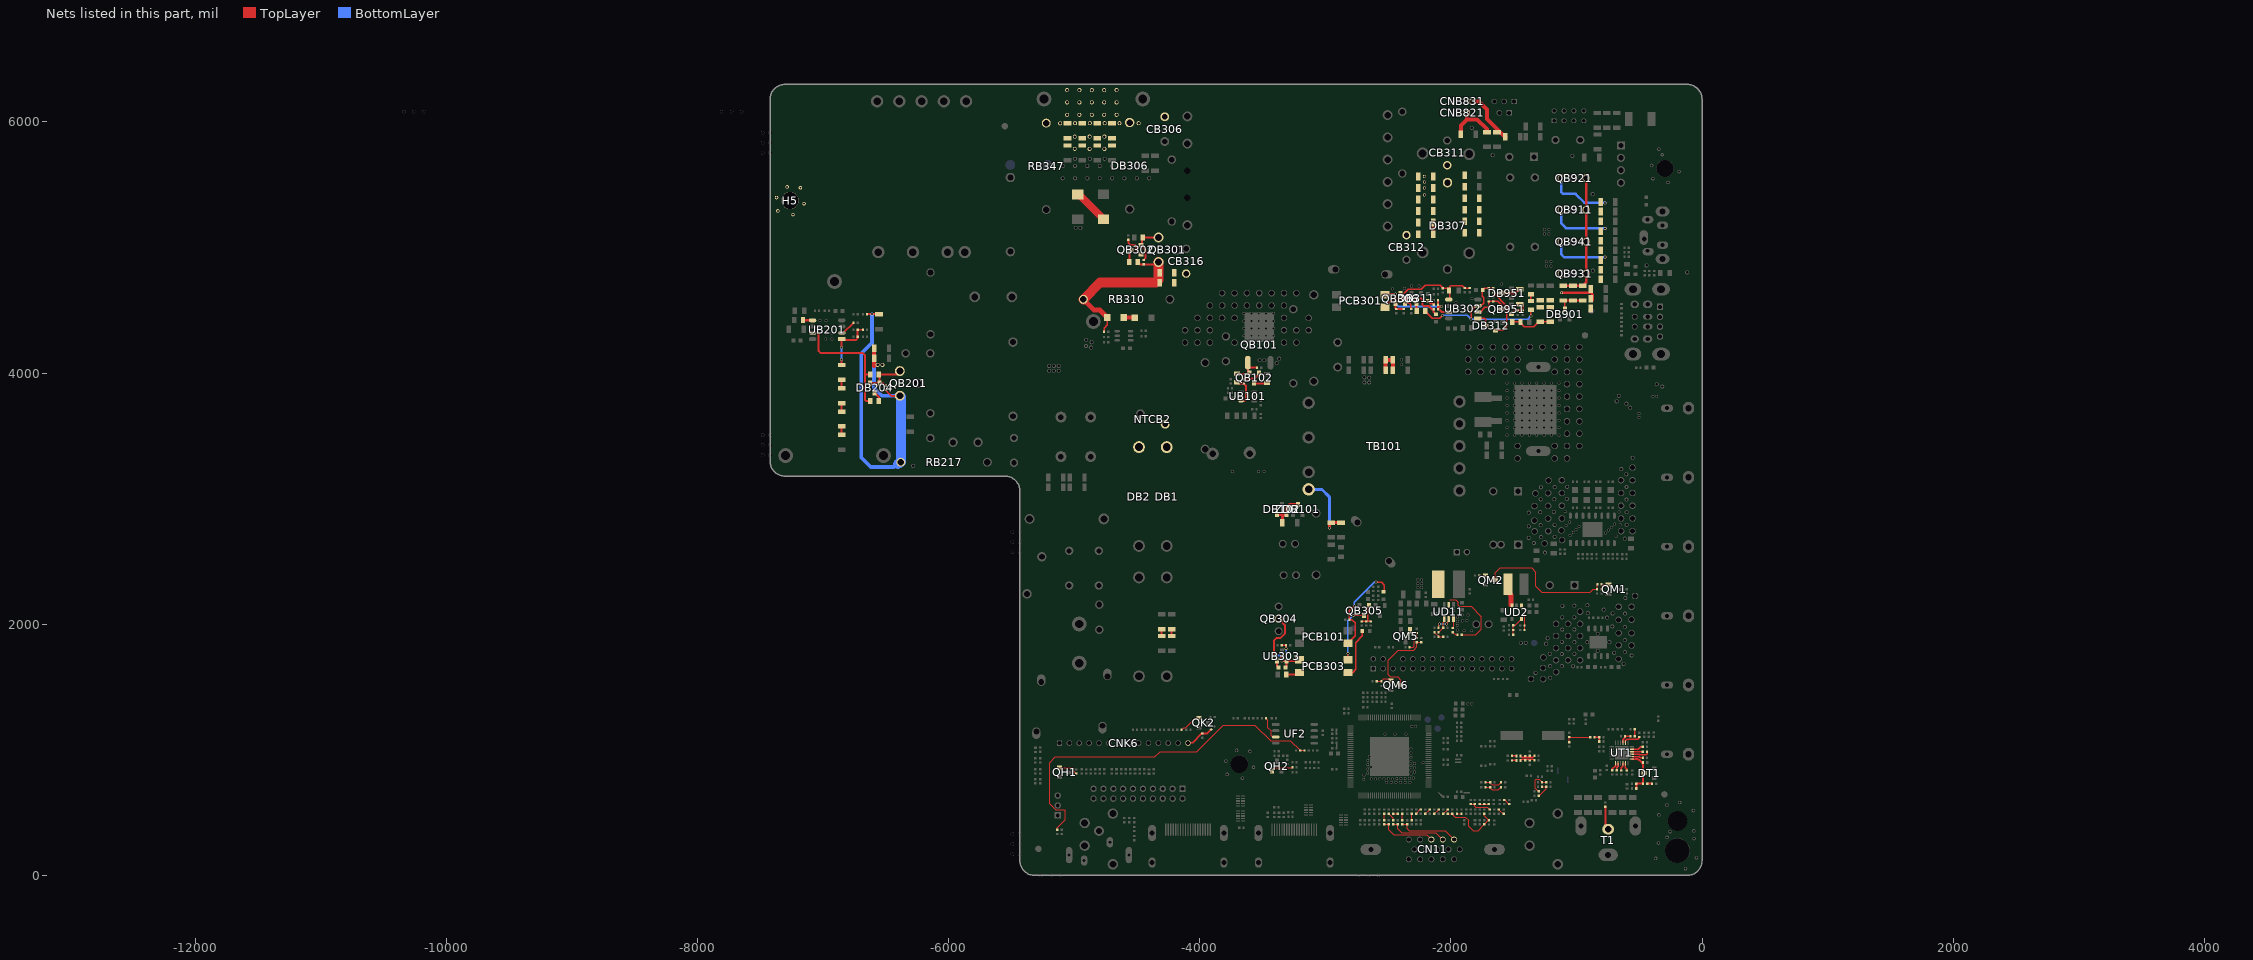
[diagram p0: the nets of this part, all layers, seen from the top]
# Altium PCB MISC84277.PcbDoc (part 12 of 15)
Units mil, origin at the board's own origin, x right, y up, seen from the top; angles counter-clockwise.
Board outline 7422.08 x 6299.21 mil, 2 copper layers (TopLayer, BottomLayer), stack 61.855 mil thick; 709 components, 395 nets, 2812 pads, 811 vias.

## Via types
v1: diameter 23.62, hole 15.75, TopLayer to BottomLayer, tented both sides, 437 vias
v2: diameter 19.68, hole 11.81, TopLayer to BottomLayer, tented both sides, 353 vias
v3: diameter 31.5, hole 23.62, TopLayer to BottomLayer, tented both sides, 16 vias
v4: diameter 31.5, hole 19.68, TopLayer to BottomLayer, tented both sides, 4 vias
v5: diameter 17.72, hole 9.84, TopLayer to BottomLayer, tented both sides, 1 vias

## Nets (pads, with @x,y where several pads share a name; then routed paths per layer and width w, separated by ;. In a path a pad name is that pad's centre, name@x,y a point inside that pad or via, vN(x,y) a via of type N, cw(c..) or ccw(c..) an arc to the next point about the centre after c; other vN are vias at no path point) (continued)
NetCB306_2: CB306.2 DB306.K pad.VIA5@-4488.19,5990.16 pad.VIA5@-4639.76,5990.16 pad.VIA5@-4663.39,6057.09 pad.VIA5@-4663.39,6155.51 pad.VIA5@-4663.39,6253.94 pad.VIA5@-4757.87,5990.16 pad.VIA5@-4761.81,6057.09 pad.VIA5@-4761.81,6155.51 pad.VIA5@-4761.81,6253.94 pad.VIA5@-4860.24,6057.09 pad.VIA5@-4860.24,6155.51 pad.VIA5@-4860.24,6253.94 pad.VIA5@-4875.98,5990.16 pad.VIA5@-4958.66,6057.09 pad.VIA5@-4958.66,6155.51 pad.VIA5@-4958.66,6253.94 pad.VIA5@-4994.09,5990.16 pad.VIA5@-5057.09,6057.09 pad.VIA5@-5057.09,6155.51 pad.VIA5@-5057.09,6253.94 pad.VIA5@-5112.75,5989.43 RB321.1 RB322.1 RB323.1 RB324.1 RB347.1
NetCB311_2: CB311.2 RB368.1 RB369.1 RB370.1 RB371.1
NetCB312_1: CB312.1 DB307.K pad.VIA5@-2212.6,5419.29 pad.VIA5@-2212.6,5474.41 pad.VIA5@-2212.6,5521.65 pad.VIA5@-2212.6,5566.93 RB331.2 RB335.2 RB368.2 RB369.2 RB370.2 RB371.2
NetCB316_1: CB316.1 RB391.1 RB392.1
NetCB321_1: CB321.1 PCB303.3 QB304.B UB303.K | length 664
  TopLayer w15.75: v1(-3404.5,1751.5) -3408.57,1751.5 -3408.57,1872.04 -3388.86,1891.75 -3356.25,1891.75 -3323.5,1924.5 -3323.5,1994 QB304.B@-3372.5,2043 ; v1(-3347.47,1705.47) UB303.K@-3309,1705.47 ; CB321.1@-3318.69,1656.76 -3309,1666.45 UB303.K@-3309,1705.47 ; PCB303.3@-3205.13,1715.5 -3215.16,1705.47 UB303.K@-3309,1705.47
  BottomLayer w15.75: v1(-3404.5,1751.5) -3362,1751.5 -3347.47,1736.97 v1(-3347.47,1705.47)
NetCB321_2: CB321.2 RB302.1 RB325.1 UB303.R | length 262.3
  TopLayer w11.81: UB303.R@-3384,1705.47 -3342.97,1746.5 v1(-3312,1746.5) ; RB325.1@-3347.27,1832.5 RB302.1@-3313.23,1832.5 -3313.23,1805.64 v1(-3312.44,1804.85)
  TopLayer w15.75: UB303.R@-3384,1705.47 -3384,1666.45 CB321.2@-3374.31,1656.76
  BottomLayer w11.81: v1(-3312.44,1804.85) -3312,1804.41 v1(-3312,1746.5)
NetCB322_1: CB322.1 RB349.2 | length 57
  TopLayer w15.75: CB322.1@-2184,4574.69 -2161.81,4552.5 RB349.2@-2136.23,4552.5
NetCB324_1: CB324.1 PCB301.2 RB348.2 RB349.1 UB302.7 | length 748.1
  TopLayer w15.75: PCB301.2@-2511.37,4613 -2522.37,4624 -2516.87,4629.5 v1(-2442.5,4629.5) ; CB324.1@-2103.77,4580 CB324.1@-2102.77,4581 -2102.77,4527.5 ; v1(-2076,4529) -2101.27,4529 -2102.77,4527.5 ; UB302.7@-2017.56,4486 -2071.5,4486 -2102.77,4517.27 -2102.77,4527.5
  BottomLayer w15.75: v1(-2442.5,4629.5) -2442.5,4556 -2415.5,4529 v1(-2076,4529) ; v1(-2076,4529) -2073.5,4531.5 -2076,4531.5 v1(-2076,4529)
NetCB326_1: CB326.1 QB306.C RB345.1 RB352.1 RB366.1 UB302.5 | length 709.2
  TopLayer w11.81: QB306.C@-2403,4632.53 -2375.97,4632.53 -2340.41,4668.09 -2234.71,4668.09 -2204.8,4698 -2084.38,4698 -2062.05,4675.67 CB326.1@-2008,4675.67 ; UB302.5@-2017.56,4586 -2008,4595.56 CB326.1@-2008,4675.67 ; RB366.1@-1887,4676.23 RB366.1@-1887.5,4676.73 ; RB352.1@-1852,4676.73 RB366.1@-1887.5,4676.73 ; CB326.1@-2008,4675.67 -2008,4692.5 -2002.99,4697.51 -1908.28,4697.51 RB366.1@-1887.5,4676.73
NetCB327_1: CB327.1 QB305.B RB385.2 RB386.1 | length 204.1
  TopLayer w11.81: RB386.1@-2711.79,2022.72 RB385.2@-2675.28,2022.72 -2655.51,2022.72 ; QB305.B@-2653.44,2148.27 -2661.42,2140.3 -2661.42,2028.62 -2655.51,2022.72 ; CB327.1@-2638.95,2022.72 -2655.51,2022.72
NetCB328_2: CB328.2 RB361.1 RB362.1 RB364.2 | length 331.9
  TopLayer w11.81: CB328.2@-1510.47,4407.5 -1454,4407.5 -1416.47,4369.97 -1340.03,4369.97 -1302.33,4407.67 RB362.1@-1288.48,4407.67 RB361.1@-1209.74,4407.67
NetCB340_1: CB340.1 QB306.B RB346.2 | length 106.3
  TopLayer w15.75: QB306.B@-2441,4554.5 -2441,4516.23 RB346.2@-2435,4510.23 CB340.1@-2375.5,4510.23
NetCB350_2: CB350.2 RB357.2 RB359.2 RB365.2 RB367.2 UB302.3 | length 1359.7
  TopLayer w11.81: RB365.2@-2203.41,4493 -2148.41,4438 -2089,4438 -2068.5,4458.5 v1(-2068.5,4458) ; v1(-1839.5,4430.5) -1839.5,4498 -1801.5,4536 UB302.3@-1785.28,4536 -1762.64,4536 -1740.4,4558.24 -1740.4,4601.55 -1750.78,4611.93 -1750.78,4658.94 CB350.2@-1734.04,4675.68 ; CB350.2@-1746.69,4660.5 -1731.51,4675.68 RB367.2@-1662.84,4675.68 ; v1(-1363.5,4456) -1363,4456.5 RB359.2@-1363,4505.91
  BottomLayer w11.81: v1(-2068.5,4458) -2068.5,4461.5 -1925.37,4461.5 -1925.25,4461.38 -1870.38,4461.38 v1(-1839.5,4430.5) -1838.66,4429.66 -1389.84,4429.66 v1(-1363.5,4456)
NetCB951_1: CB951.1 QB951.B RB951.2 RB952.1 | length 149.8
  TopLayer w15.75: QB951.B@-1517.68,4471.38 -1492.23,4496.83 RB951.2@-1469.49,4496.83 CB951.1@-1430.12,4496.83 RB952.1@-1430.12,4548.5
NetCD2_1: CD2.1 LD12.1 UD11.2 | length 597.1
  TopLayer w8: -2008.7,2194.85 -1960.12,2194.85 -1940.63,2175.35 -1940.63,2150.4 -1933.6,2143.37 -1840.21,2143.37 -1757.87,2061.04 -1757.87,1958.66 -1801.1,1915.44 CD2.1@-1913.8,1915.44
NetCD2_2: CD2.2 RD15.2 | length 45.5
  TopLayer w8: RD15.2@-1984.25,1936.02 -1963.67,1915.44 CD2.2@-1947.26,1915.44
NetCD7_1: CD7.1 RD13.2 UD11.4 | length 126.4
  TopLayer w7: RD13.2@-2098.27,1936 -2096.73,1936 CD7.1@-2060.73,1972
  TopLayer w8: CD7.1@-2060.73,1972 -2060.73,2014.27 -2054.11,2020.89 UD11.4@-2054.11,2043.23
NetCD13_2: CD13.2 RD6.1 RD7.2 UD2.5 | length 159.3
  TopLayer w8: CD13.2@-1503.27,1917 RD7.2@-1503.27,1991 -1488.72,1991 -1439.3,2040.42 UD2.5@-1439.3,2041.25
NetCD17_2: CD17.2 RD8.2 UD2.1 | length 209.1
  TopLayer w8: UD2.1@-1439.3,2149.52 -1439.3,2146.89 -1410.39,2117.98 -1410.39,1957.87 RD8.2@-1414.27,1954
NetCF26_2: CF26.2 RF12.1 | length 36
  TopLayer w7: CF26.2@-1952,490.27 RF12.1@-1916,490.27
NetCF31_2: CF31.2 RF16.1 | length 37
  TopLayer w6: CF31.2@-2460,491.27 RF16.1@-2423,491.27
NetCF32_1: CF32.1 CF33.2 CF38.2 | length 221
  TopLayer w6: CF38.2@-1059.05,1060.31 CF32.1@-1059.06,1101.65 -1057.4,1100 -1012.6,1100 ; -1023.23,1100 -1012.6,1100 ; CF33.2@-890.73,1100 -1012.6,1100
NetCF33_1: CF33.1 CF39.2 LF7.1 | length 75.5
  TopLayer w12: CF33.1@-857.28,1100 CF39.2@-818.73,1100 LF7.1@-818.73,1063
NetCF34_2: CF34.2 RF19.1 | length 50.9
  TopLayer w6: CF34.2@-2205,490.27 -2203.73,490.27 -2170.27,523.73 RF19.1@-2168,523.73
NetCI1_2: CI1.2 RI3.1 | length 49.9
  TopLayer w6: CI1.2@-2060,490.27 -2026.54,523.73 RI3.1@-2024,523.73
NetCI2_1: CI2.1 RI1.2 RI2.2 RI3.2 RI18.2 | length 507
  TopLayer w8: RI3.2@-2024,490.27 -1992.27,490.27 -1966,464 -1884.62,464 -1858,437.38 -1858,390.97 -1823.08,356.06 -1783.84,356.06 -1734,405.9 RI1.2@-1734,406.27 RI18.2@-1701.54,438.73 ; RI2.2@-1734,490.27 -1734,475 -1697.73,438.73 RI18.2@-1697,438.73
NetCI3_2: CI3.2 RI4.1 RI5.2 | length 179.6
  TopLayer w8: CI3.2@-1844,567.27 RI5.2@-1809,567.27 -1809,551 -1802,544 -1712.27,544 RI4.1@-1692,523.73
NetCI4_2: CI4.2 RI6.1 RI7.1 | length 74
  TopLayer w8: CI4.2@-1772,567.27 RI6.1@-1698,567.27
NetCI5_2: CI5.2 RI8.1 RI9.2 | length 201.7
  TopLayer w8: CI5.2@-1301.27,669 -1303,669 -1329,695 -1329,759 -1324,764 -1295,764 -1274.27,743.27 RI9.2@-1274.27,743 RI8.1@-1240.73,743
NetCI6_2: CI6.2 RI10.1 RI11.1 | length 135.7
  TopLayer w8: CI6.2@-1301.27,633 -1296,633 -1240.73,688.27 RI10.1@-1240.73,707 RI11.1@-1274.27,707
NetCI7_2: CI7.2 RI12.2 | length 49.9
  TopLayer w8: CI7.2@-2278,491.27 -2244.54,524.73 RI12.2@-2242,524.73
NetCI9_2: CI9.2 RI14.1 | length 51.5
  TopLayer w8: RI14.1@-2314,439.73 CI9.2@-2314,491.27
NetCI11_2: CI11.2 RI16.1 | length 49.9
  TopLayer w8: CI11.2@-2132,490.27 -2131.73,490.27 -2098.27,523.73 RI16.1@-2096,523.73
NetCK1_2: CK1.2 CNK6.14 RK1.2 | length 226
  TopLayer w15: CNK6.14@-4091.3,1056.4 -4057.05,1056.4 -3983.51,1129.93 CK1.2@-3980.6,1129.93 -3940.71,1129.93 RK1.2@-3908.91,1161.73
NetCM1_2: CM1.2 QM1.G RM2.2 | length 93.9
  TopLayer w8: CM1.2@-798,2278.73 -800.27,2281 RM2.2@-800.27,2317 -747.84,2317 QM1.G@-746.24,2315.4
NetCM3_1: CM3.1 CM7.2 QM5.G RM7.2 | length 231.2
  TopLayer w8: CM7.2@-2329.27,1816 -2301,1816 -2293,1824 -2293,1884 -2286.27,1890.73 RM7.2@-2272,1890.73 CM3.1@-2272,1930.27 -2306.27,1930.27 -2325.6,1949.6 QM5.G@-2325.6,1956.24
NetCN11_1: CN11.1 RV1.2 RV2.2 | length 481.3
  TopLayer w8: RV1.2@-2387,406.27 RV2.2@-2350,406.27 -2350,373 -2334,357 -2046.72,357 CN11.1@-1975.2,285.48
NetCN11_2: CN11.2 RV3.2 RV5.2 | length 466.5
  TopLayer w8: RV3.2@-2460,406.27 RV5.2@-2423,406.27 -2423,372 -2391,340 -2119.88,340 CN11.2@-2065.36,285.48 CN11.2@-2064.15,286.68
NetCN11_3: CN11.3 RV9.2 RV11.2 | length 452.5
  TopLayer w8: RV9.2@-2532,406.27 RV11.2@-2496,406.27 -2496,362 -2456,322 -2192.03,322 CN11.3@-2155.51,285.48
NetCNB821_1: CNB821.1 JB102.1 JB103.2 | length 430.8
  TopLayer w31.5: JB102.1@-1920.66,5901.27 -1920.66,5971.83 -1871.77,6020.71 CNB821.1@-1871.77,6072.15 ; -1871.51,6020.97 -1792.57,6020.97 -1714.4,5942.8 JB103.2@-1714.4,5919.26
  BottomLayer w31.5: -1871.77,6045.55 CNB821.1@-1871.77,6072.15
NetCNB831_1: CNB831.1 JB106.2 JB107.2 | length 427
  TopLayer w31.5: CNB831.1@-1832.4,6163.14 -1777.31,6163.14 -1713.94,6099.77 -1713.94,6024.54 -1571.1,5881.7 JB107.2@-1566.03,5881.7
NetCO1_2: CO1.2 RO1.2 | length 50.9
  TopLayer w8: CO1.2@-1574,600.73 -1572.73,600.73 -1539.27,567.27 RO1.2@-1537,567.27
NetCO4_2: CO4.2 RO5.2 | length 50.4
  TopLayer w8: CO4.2@-1618,523.73 -1585.53,491.27 RO5.2@-1581,491.27
NetCO6_2: CO6.2 RO9.2 RO10.1 | length 2889.3
  TopLayer w7: -3422.88,1072.31 -3278.55,1072.31 RO10.1@-3200.67,994.42 RO9.2@-3166.73,994.42
  TopLayer w8: CO6.2@-5136.7,363.53 -5136.7,377.5 -5073,441.2 -5073,513.17 -5081.6,521.77 -5149.05,521.77 -5196.5,569.22 -5196.5,897.93 -5151.59,942.84 -4358.61,942.84 -4315.26,986.2 -4022.66,986.2 -3811.7,1197.16 -3560.91,1197.16 -3435.57,1071.81 -3422.88,1071.81
NetCT10_1: CT10.1 RT1.1 RT9.1 RT12.2 | length 118.3
  TopLayer w12: RT1.1@-1445.44,951.3 -1434.93,940.79 -1345.67,940.79 RT9.1@-1335.67,950.79
NetCT11_2: CT11.2 UT1.20 | length 61.9
  TopLayer w10: CT11.2@-679.97,837.09 -679.97,857.36 -669.45,867.88 UT1.20@-669.45,894.6
NetCT12_1: CT12.1 UT1.19 | length 68.6
  TopLayer w10: CT12.1@-715.97,837.09 -715.97,847.86 -689.13,874.69 UT1.19@-689.13,894.6
NetCT13_2: CT13.2 CT17.2 DT1.2 LT3.2 LT6.1 UT1.1 | length 351
  TopLayer w10: UT1.1@-559.21,926.1 -531.21,926.1 -530.97,925.86
  TopLayer w15.8: -530.97,925.86 -521.62,925.86 cw(c-521.62,890.72) -496.78,915.57 -481.56,900.35 cw(c-507.5,874.41) -470.82,874.41 CT17.2@-470.82,730.26 ; LT3.2@-524,692.26 CT13.2@-524,730.27 CT17.2@-470.82,730.26
NetCT17_1: CT17.1 LT9.2 | length 38.6
  TopLayer w15.8: CT17.1@-437.35,730.26 LT9.2@-398.74,730.27
NetCT20_1: CT20.1 RT1.2 | length 40.8
  TopLayer w12: CT20.1@-1516.44,951.29 RT1.2@-1481.2,951.29 ; RT1.2@-1478.91,951.3 RT1.2@-1481.2,951.29 ; RT1.2@-1478.91,953.59 RT1.2@-1481.2,951.29
NetCT21_1: CT21.1 UT1.5 | length 94.1
  TopLayer w10: UT1.5@-559.21,1004.84 -507.2,1004.84 -489.62,1022.41 CT21.1@-472.35,1022.41
NetCT23_1: CT23.1 RT14.2 | length 37.5
  TopLayer w12: CT23.1@-1516.44,914.79 RT14.2@-1478.91,914.8
NetCT24_2: CT24.2 RT10.1 RT12.1 RT14.1 | length 123.5
  TopLayer w12: RT14.1@-1445.44,914.8 RT14.1@-1444.45,915.79 ; RT14.1@-1445.44,915.79 RT14.1@-1444.45,915.79 ; RT14.1@-1440.9,915.79 RT14.1@-1444.45,915.79 ; RT12.1@-1408.44,922.29 RT12.1@-1406.94,923.79 ; RT10.1@-1335.67,915.79 -1343.67,923.79 RT12.1@-1406.94,923.79 ; RT14.1@-1444.45,915.79 -1436.45,923.79 RT12.1@-1406.94,923.79
NetCT25_1: CT25.1 UT1.8 | length 142.5
  TopLayer w10: UT1.8@-610.39,1056.02 -610.39,1072.21 -597.69,1084.91 -511.69,1084.91 -498.92,1097.68 CT25.1@-498.92,1101.95
NetCT26_2: CT26.2 RT11.2 UT1.9 | length 101.2
  TopLayer w10: UT1.9@-630.08,1056.02 -630.08,1081.52 -613.19,1098.41 CT26.2@-613.19,1109.68
  TopLayer w12: CT26.2@-610.19,1109.68 RT11.2@-569.65,1109.68
NetCT29_2: CT29.2 RT11.1 | length 39
  TopLayer w10: RT11.1@-538.19,1112.68 -538.19,1151.68
NetCT40_1: CT40.1 T1.1 | length 181.4
  TopLayer w15.8: T1.1@-770.21,365.11 CT40.1@-770.21,546.53
NetCV1_2: CV1.2 RV1.1 | length 51.5
  TopLayer w8: RV1.1@-2387,439.73 CV1.2@-2387,491.27
NetCV3_2: CV3.2 RV3.1 | length 66.4
  TopLayer w8: CV3.2@-2496,491.27 -2496,489 -2460,453 RV3.1@-2460,439.73
NetCV5_1: CV5.1 RV4.2 RV6.1 | length 144.8
  TopLayer w8: CV5.1@-1725.27,701 -1686.73,701 -1686.73,694.73 -1672,680 -1622.35,680 -1601.73,700.62 RV6.1@-1601.73,701.01
NetCV6_1: CV6.1 RV7.1 RV8.1 | length 146.3
  TopLayer w8: CV6.1@-1725.27,739.99 -1685.72,739.99 -1685.72,734.72 -1670.84,719.84 -1665.86,719.84 -1665.7,720 -1618.73,720 RV7.1@-1598.73,740
NetCV7_2: CV7.2 RV9.1 | length 51.5
  TopLayer w8: RV9.1@-2532,439.73 CV7.2@-2532,491.27
NetDB1_K: DB1.K DB2.K NTCB2.2@-4276.07,3592.66
NetDB102_1: DB102.1 DB102.3 RB110.1 ZDB101.2 | length 292.5
  TopLayer w23.62: DB102.1@-3384.5,2875.5 DB102.3@-3309.5,2875.5 -3309.5,2928 -3283.97,2953.53 ZDB101.2@-3219,2953.53 ; RB110.1@-3342.06,2807.5 -3342.06,2871.44
NetDB202_K: DB202.K DB203.A | length 287.6
  TopLayer w59.06: DB202.K@-4971.94,5422.83 -4964.76,5422.83 DB203.A@-4766.44,5224.51
NetDB204_1: DB204.1 DB204.3 QB201.G RB212.2 RB214.2 | length 377
  TopLayer w15.75: DB204.3@-6627.42,3921.88 DB204.1@-6552.42,3921.88 ; RB212.2@-6555.83,3989.81 -6415.82,3989.81 QB201.G@-6389.31,4016.31 ; RB212.2@-6552.42,3986.41 DB204.1@-6552.42,3921.88 ; RB214.2@-6502.12,3898.61 -6525.39,3921.88 DB204.1@-6552.42,3921.88
NetDB204_2: DB204.2 RB213.2 | length 80
  TopLayer w15.75: DB204.2@-6589.92,3843.85 -6555.83,3809.75 RB213.2@-6555.83,3777.97
NetDB311_2: DB311.2 RB365.1 | length 51.4
  TopLayer w15.75: RB365.1@-2275,4505.09 DB311.2@-2275,4556.47
NetDB312_1: DB312.1 RB367.1 | length 420.1
  TopLayer w11.81: RB367.1@-1662.84,4642.21 -1662.19,4642.21 -1554,4534.02 -1554,4373 -1587.5,4339.5 DB312.1@-1645.5,4339.5
NetDB312_3: DB312.3 UB302.1 | length 126.3
  TopLayer w11.81: UB302.1@-1773.27,4436 UB302.1@-1785.28,4436 -1734.5,4436 -1723.53,4425.03 DB312.3@-1723.53,4377
NetDB370_A: DB370.A QB301.S RB305.2 RB308.2 RB309.1 RB310.2 RB391.2 RB392.2 | length 1357.3
  TopLayer w11.81: RB305.2@-4762.14,4330.86 -4762.14,4357.94 -4736.2,4383.88 DB370.A@-4736.2,4443.16
  TopLayer w15.75: RB308.2@-4493.41,4883.5 -4476.67,4866.77 RB309.1@-4448,4866.77 -4345.48,4866.77 QB301.S@-4328.3,4883.94
  TopLayer w39.37: RB310.2@-4927.09,4587.13 -4841.94,4501.97 -4795,4501.97 DB370.A@-4736.2,4443.16
  TopLayer w78.74: RB310.2@-4927.09,4587.13 -4793.75,4720.47 -4350.39,4720.47 -4328.3,4742.56 QB301.S@-4328.3,4883.94
NetDB370_K: DB370.K DB371.A | length 75.1
  TopLayer w31.5: DB370.K@-4602.31,4441.16 DB370.K@-4604.31,4443.16 -4532.7,4443.16 DB371.A@-4532.2,4442.66
NetDB901_2: DB901.2 RB901.2 RB902.2 RB903.2 | length 215.2
  TopLayer w11.81: DB901.2@-1093.5,4507.03 RB902.2@-1093.5,4567.79
  TopLayer w19.68: RB902.2@-1103.84,4578.13 RB903.2@-949.39,4578.13
NetDB951_2: DB951.2 RB952.2 | length 158.8
  TopLayer w19.68: DB951.2@-1595.71,4636.79 -1490.5,4636.79 RB952.2@-1452.6,4674.69
NetH5_0: H5.0 H5.1 H5.2 H5.3 H5.4 H5.5 H5.6
NetLD2_1: LD2.1 UD2.3 | length 174.6
  TopLayer w40: LD2.1@-1546.96,2319 -1546.96,2257.96 -1521.7,2232.7 UD2.3@-1521.7,2154.85
NetLT1_2: LT1.2 UT1.23 | length 65
  TopLayer w10: UT1.23@-610.39,896.95 UT1.23@-610.39,894.6 -610.39,858.18 -600.14,847.93 LT1.2@-600.14,836.15
NetLT2_1: LT2.1 UT1.22 | length 63.7
  TopLayer w10: LT2.1@-642.74,836.14 -642.74,856.58 -630.08,869.25 UT1.22@-630.08,894.6
NetLT8_1: LT8.1 UT1.2 | length 97.8
  TopLayer w10: UT1.2@-559.21,945.78 -500.26,945.78 -491.87,937.39 LT8.1@-471.44,937.39 LT8.1@-476.05,932.78
NetLT10_1: LT10.1 UT1.4 | length 87.1
  TopLayer w10: UT1.4@-559.21,985.15 -472.41,985.15 LT10.1@-472.21,985.36
NetLT10_2: LT10.2 UT1.3 | length 139.1
  TopLayer w10: UT1.3@-559.21,965.47 -501.08,965.47 -497.47,961.86 -442.97,961.86 -438.46,966.37 LT10.2@-438.46,981.4
NetPCB101_1: PCB101.1 RB131.2 RB132.1 | length 766.4
  TopLayer w11.81: PCB101.1@-2820.87,1849.5 -2761.81,1908.56 -2761.81,1968.5 -2761.81,2009.84 -2789.37,2037.4 RB132.1@-2808.07,2037.4 -2808.07,2107.27 v1(-2769.68,2145.66) ; v1(-2596.46,2334.65) -2553.15,2334.65 -2529.53,2311.02 -2529.53,2267.97 RB131.2@-2537.4,2260.09
  BottomLayer w11.81: v1(-2769.68,2145.66) -2769.68,2175.2 -2610.24,2334.65 v1(-2596.46,2334.65)
NetPCB301_1: PCB301.1 RB348.1 RB350.1 | length 526.5
  TopLayer w15.75: PCB301.1@-2522.37,4524 -2522.37,4531.01 -2458.38,4595 -2237,4595 -2228.5,4586.5 -2228.5,4546 -2218.5,4536 -2178.9,4536 -2150.9,4508 RB348.1@-2137.23,4508 -2137.23,4485.01 RB350.1@-2119.5,4467.28
NetPCB303_1: PCB303.1 RB384.2 | length 400
  TopLayer w11.81: PCB303.1@-2820.87,1615.5 -2782.14,1615.5 -2757.91,1639.73 -2757.91,1854.3 -2705.06,1907.15 RB384.2@-2705.06,1944.88
NetPCB303_2: PCB303.2 QB305.C | length 459.2
  TopLayer w11.81: PCB303.2@-2820.87,1715.5 v1(-2820.87,1765.74) ; v1(-2778.19,2070.24) QB305.C@-2691.45,2070.24
  BottomLayer w11.81: v1(-2820.87,1765.74) -2820.87,2027.55 v1(-2778.19,2070.24)
NetPCB303_4: PCB303.4 RB326.2 | length 112.7
  TopLayer w15.75: RB326.2@-3311.41,1600 -3220.63,1600 PCB303.4@-3205.13,1615.5
NetQB101_G: QB101.G QB102.E RB106.2 RB109.1 | length 219.3
  TopLayer w15.75: RB106.2@-3702.9,3993.85 -3621.5,3993.85 -3618.1,3997.25 -3618.1,4052.5 -3608.35,4042.75 RB109.1@-3544.28,4042.75
NetQB102_B: QB102.B RB107.2 | length 140.4
  TopLayer w15.75: RB107.2@-3650.9,3950.49 -3644.39,3957 -3565.16,3957 QB102.B@-3528.4,3993.76
NetQB102_C: QB102.C RB108.1 | length 94.6
  TopLayer w15.75: QB102.C@-3566.4,3915.73 RB108.1@-3471.83,3915.73
NetQB201_S: pad.VIA5@-6528,4065 pad.VIA5@-6566,4065 QB201.S RB214.1 RB215.2 RB217.2 RB218.2 RB223.2 RB224.2 | length 2877.7
  TopLayer w15.75: RB215.2@-6649.66,4468.8 v1(-6612.5,4468.8) -6555.2,4468.8 RB218.2@-6555,4469 ; RB214.1@-6502.12,3865.15 -6456.44,3819.46 QB201.S@-6389.31,3819.46
  TopLayer w31.5: -6593.43,4056.43 RB224.2@-6593.43,4196.82
  BottomLayer w31.5: v1(-6612.5,4468.8) -6612.5,4241.5 -6696.5,4157.5 -6696.5,3327 -6621,3251.5 -6441,3251.5 -6402,3290.5 -6389.18,3290.5 RB217.2@-6380.99,3290.5 ; -6593.43,4056.43 -6593.43,3882.43 -6530.46,3819.46 QB201.S@-6389.31,3819.46
  BottomLayer w78.74: RB217.2@-6405.5,3274.18 -6389.18,3290.5 RB217.2@-6380.99,3298.69 ; QB201.S@-6389.31,3819.46 -6380.99,3811.14 RB217.2@-6380.99,3298.69 ; RB217.2@-6380.99,3290.5 RB217.2@-6380.99,3298.69
NetQB301_G: QB301.G QB302.E RB306.2 RB309.2 | length 313
  TopLayer w15.75: QB302.E@-4470,5019 -4433,4982 -4433,4915.23 RB309.2@-4448,4900.23 ; QB302.E@-4460.63,5022.52 RB306.2@-4460.63,5068.9 ; RB306.2@-4455.87,5079.5 QB301.G@-4329.59,5079.5
NetQB302_B: QB302.B RB307.2 | length 180.2
  TopLayer w15.75: RB307.2@-4569.47,5062.77 -4569.47,5037.47 -4553.5,5021.5 -4519,5021.5 -4507.5,5010 -4507.5,4981.5 QB302.B@-4470,4944
NetQB302_C: QB302.C RB308.1 | length 104.1
  TopLayer w15.75: RB308.1@-4561.59,4883.5 -4561.59,4968.44 QB302.C@-4548.03,4982
NetQB306_E: QB306.E RB356.1 | length 88.5
  TopLayer w11.81: QB306.E@-2366,4551.5 QB306.E@-2366,4554.5 -2328.5,4554.5 -2319.5,4545.5 RB356.1@-2319.5,4510.23
NetQB911_B: QB911.B QB921.B QB931.B QB941.B RB901.1 RB902.1 RB903.1 | length 1011.6
  TopLayer w19.68: RB902.1@-1103.84,4696.24 -949.39,4696.24 -924.08,4721.55 QB921.B@-924.08,5542.89
NetQB911_E: QB911.E RB911.2 RB912.2 RB913.2 | length 479.4
  BottomLayer w19.68: QB911.E@-1120.92,5307.26 -1120.92,5191.42 -1084,5154.5 v1@-772.67,5154.5
  other v1: -771.37,5149.9
NetQB921_E: QB921.E RB921.2 RB922.2 RB923.2 | length 486.9
  BottomLayer w19.68: QB921.E@-1120.92,5542.89 -1120.92,5439.92 -1108.5,5427.5 -1007.87,5427.5 -936.67,5356.3 -885.83,5356.3 ; -885.8,5356.27 v1(-771.68,5356.27)
NetQB931_E: QB931.E RB931.2 RB932.2 RB933.2 | length 300.8
  TopLayer w19.68: v1(-1119.5,4640) -886,4640 -871.38,4625.38 RB932.2@-871.38,4578.76
NetQB941_E: QB941.E RB941.2 RB942.2 RB943.2 | length 485.6
  BottomLayer w19.68: QB941.E@-1120.92,5071.63 -1120.92,4944.92 -1098.5,4922.5 -772.37,4922.5 v1(-771.65,4923.22)
NetQH1_B: QH1.B RH7.1 | length 161.9
  TopLayer w5: QH1.B@-5116.3,857.58 -5013.58,857.58 -5004.9,848.9 -5004.9,829.97 RH7.1@-4985.1,810.17
NetQH2_B: QH2.B RH16.1 | length 174.2
  TopLayer w5: QH2.B@-3425.2,830.9 -3398.01,858.08 -3264.95,858.08 RH16.1@-3263.03,860
NetQK2_B: QK2.B RK20.1 | length 176.5
  TopLayer w5: RK20.1@-4145.87,1160 -4128.52,1177.35 -4110.85,1177.35 -4036.4,1251.8 QK2.B@-4007.4,1251.8
NetQM2_B: QM2.B RM4.1 | length 50.9
  TopLayer w8: RM4.1@-1774.27,2388 -1725.5,2388 QM2.B@-1724,2389.5
NetQM2_C: QM2.C RM1.1 RM2.1 | length 1079.8
  TopLayer w6: QM2.C@-1645.97,2351.5 -1645.97,2411.03 -1609,2448 -1357.72,2448 -1324.8,2415.09 -1324.8,2303.15 -1275.4,2253.75 -889.95,2253.75 -864.97,2278.73 RM1.1@-837,2278.73 -833.73,2282 RM2.1@-833.73,2317
NetQM6_B: QM6.B RM8.2 RM10.1 | length 127.6
  TopLayer w6: RM10.1@-2553.73,1545 -2553.73,1548.27 -2537,1565 -2490.5,1565 QM6.B@-2478,1552.5
  TopLayer w8: RM8.2@-2590.27,1545 RM10.1@-2553.73,1545
NetQM6_C: QM6.C RM5.1 RM7.1 | length 621
  TopLayer w6: QM6.C@-2399.97,1514.5 -2399.97,1554.97 -2425,1580 -2484,1580 -2500.6,1596.6 -2500.6,1711.4 -2418,1794 -2298,1794 -2272,1820 RM7.1@-2272,1857.27 RM5.1@-2235,1857.27
NetRB101_2: RB101.2 RB102.1 | length 54.2
  TopLayer w15.75: RB102.1@-4304.29,1906.46 RB101.2@-4304.29,1960.65
NetRB106_1: RB106.1 RB107.1 UB101.6 | length 232
  TopLayer w15.75: RB106.1@-3702.9,3925.67 -3694.26,3917.03 RB107.1@-3650.9,3917.03 -3633.86,3899.99 -3633.86,3791.34 -3648.1,3777.1 UB101.6@-3671.65,3777.1
NetRB114_2: RB114.2 RB115.2 TB101.6@-3133.09,3074.01 | length 564.7
  TopLayer w23.62: v1(-2969,2766.5) -2969,2795.05 RB114.2@-2954.5,2809.55 RB115.2@-2875.97,2809.55
  BottomLayer w23.62: TB101.6@-3133.09,3074.01 -3027.91,3074.01 -2969,3015.11 v1(-2969,2766.5)
NetRB141_1: RB141.1 RB142.2 | length 54.2
  TopLayer w15.75: RB142.2@-4224.49,1906.46 RB141.1@-4224.49,1960.65
NetRB144_2: RB144.2 RB145.1 RB146.2 RB147.1 | length 224.5
  TopLayer w31.5: RB146.2@-2520.27,4022 RB144.2@-2520.27,4105.75 RB145.1@-2463.31,4105.75 RB147.1@-2463.31,4022
NetRB201_2: RB201.2 RB202.1 | length 67.5
  TopLayer w15.75: RB201.2@-6853,3507.81 RB202.1@-6853,3575.28
NetRB202_2: RB202.2 RB203.1 | length 67.5
  TopLayer w15.75: RB202.2@-6853,3693.39 RB203.1@-6853,3760.86
NetRB203_2: RB203.2 RB204.1 | length 67.5
  TopLayer w15.75: RB203.2@-6853,3878.97 RB204.1@-6853,3946.44
NetRB204_2: RB204.2 RB205.2 RB206.1 RB221.2 UB201.1 | length 451.3
  TopLayer w15.75: RB204.2@-6853,4064.55 v1(-6853,4110) ; v1(-6853,4205) -6853,4269.08 UB201.1@-6851.71,4270.37 -6845.63,4264.28 -6736.72,4264.28 -6724.46,4276.54 RB205.2@-6724.46,4290 RB206.1@-6724.46,4345.31 RB221.2@-6683.12,4345.31
  BottomLayer w15.75: v1(-6853,4110) v1(-6853,4205)
NetRB209_1: RB209.1 UB201.5 | length 77
  TopLayer w19.68: RB209.1@-7160.53,4421.55 -7159.35,4420.37 UB201.5@-7084,4420.37
NetRB212_1: RB212.1 RB213.1 UB201.7 | length 1014.9
  TopLayer w15.75: UB201.7@-7084,4320.37 -7048.5,4320.37 -7036.5,4308.37 -7036.5,4176.26 -7021.74,4161.5 -6685.12,4161.5 -6667,4143.38 -6667,3983.5 ; RB213.1@-6624.02,3777.97 -6655.47,3777.97 -6667,3789.5 -6667,3983.5 ; RB212.1@-6624.02,3989.81 -6660.69,3989.81 -6667,3983.5
NetRB226_2: RB226.2 UB201.2 | length 113.5
  TopLayer w15.75: UB201.2@-6838.17,4320.37 RB226.2@-6757.93,4400.61
NetRB317_1: pad.VIA5@-4759.84,5785.43 pad.VIA5@-4759.84,5883.86 pad.VIA5@-4877.95,5785.43 pad.VIA5@-4877.95,5883.86 pad.VIA5@-4996.06,5785.43 pad.VIA5@-4996.06,5883.86 RB317.1 RB318.1 RB319.1 RB320.1 RB321.2 RB322.2 RB323.2 RB324.2
NetRB328_2: RB328.2 RB329.1 RB332.2 RB333.1
NetRB329_2: RB329.2 RB330.1 RB333.2 RB334.1
NetRB330_2: RB330.2 RB331.1 RB334.2 RB335.1 | length 91.8
  TopLayer w31.5: RB335.1@-2141.01,5107.06 RB331.1@-2141.01,5198.86
NetRB358_2: RB358.2 RB359.1 | length 55.3
  TopLayer w11.81: RB359.1@-1363,4574.09 RB358.2@-1363,4629.41
NetRB360_1: RB360.1 RB361.2 RB362.2 RB363.1
NetRD1_2: RD1.2 UD11.5 | length 135.2
  TopLayer w8: RD1.2@-2098.27,1973 -2098.27,1994 v1(-2090.27,2002) ; v1@-2037,2002 -2016.7,2022.3 UD11.5@-2016.7,2043.23
  BottomLayer w8: v1(-2090.27,2002) v1@-2037,2002
  other v1: -2037,2001
NetRD12_1: RD12.1 RD13.1 RD16.2 | length 84.9
  TopLayer w7: RD13.1@-2131.73,1936 RD16.2@-2098.27,1902.54 ; RD16.2@-2098.27,1900 RD12.1@-2060.73,1900
NetRD15_1: RD15.1 UD11.6 | length 75.8
  TopLayer w8: RD15.1@-1984.25,1969.49 -1979.3,1974.44 UD11.6@-1979.3,2043.23
NetRF2_1: RF2.1 UF2.3 | length 201.1
  TopLayer w6: RF2.1@-3472.27,1251 -3457.6,1236.33 -3457.6,1176.47 -3433.07,1151.94 -3433.07,1112.17 -3422.9,1102 UF2.3@-3395.54,1102 UF2.3@-3395.54,1106.27
OCP: CB305.1 QB951.C RB354.1 RB355.1 UB302.2 | length 298.2
  TopLayer w11.81: UB302.2@-1785.28,4486 -1766.58,4486 -1729.52,4523.06 RB354.1@-1702.21,4523.06 ; RB354.1@-1704.57,4520.7 RB354.1@-1702.21,4523.06 ; QB951.C@-1595.71,4509.38 -1595.71,4540.21 -1626.54,4571.04 CB305.1@-1699.45,4571.04 -1699.45,4525.82 RB354.1@-1702.21,4523.06